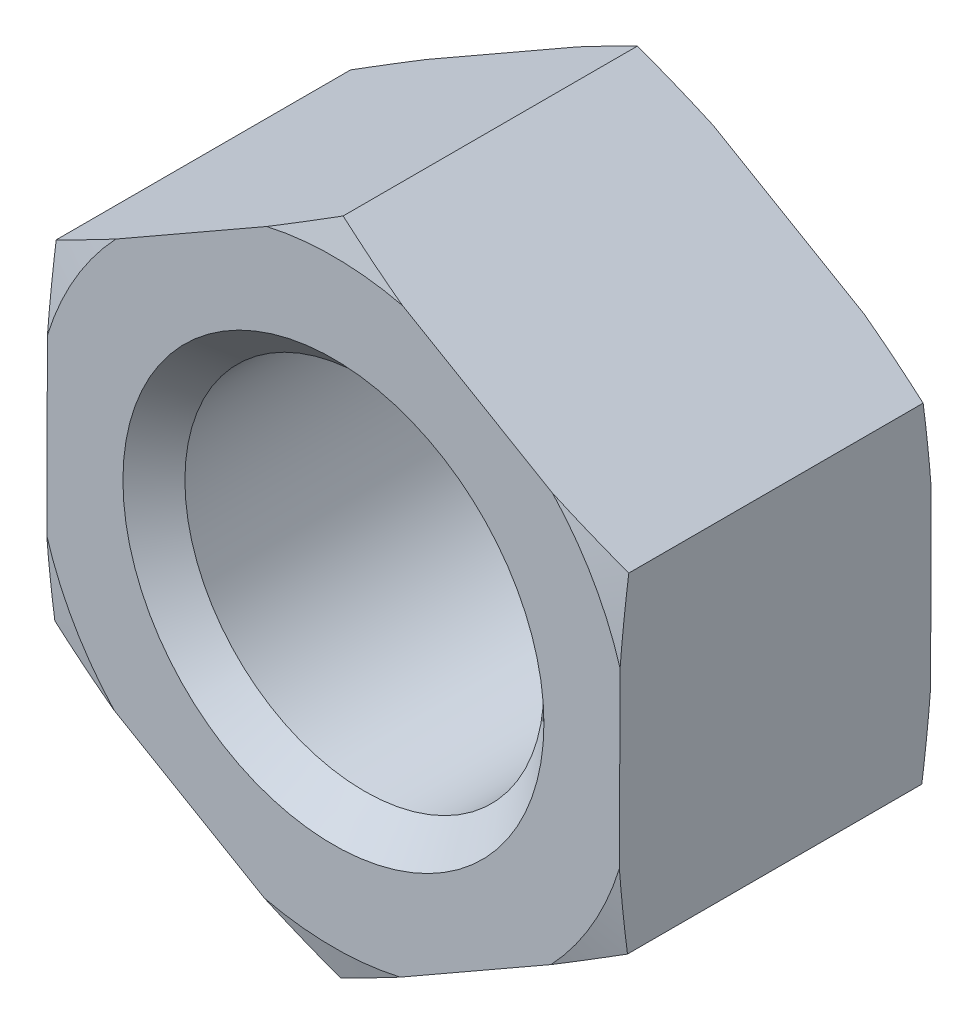
SolidWorks part; units mm, degrees
extrude "Base-Extrude" add sketch "Sketch1" along normal blind 5.2
sketch "Sketch1" plane through (0, 0, 0) normal (0, 0, 1) x (1, 0, 0)
  line L0 (-26.8088, 0) -> (37.1748, 0) construction
  line L1 (0, 25.0215) -> (0, -25.0215) construction
  line L3 (0.0217, 5.525) -> (-4.7739, 2.7813)
  line L4 (-4.7739, 2.7813) -> (-4.7956, -2.7437)
  line L5 (-4.7956, -2.7437) -> (-0.0217, -5.525)
  line L6 (-0.0217, -5.525) -> (4.7739, -2.7813)
  line L7 (4.7739, -2.7813) -> (4.7956, 2.7437)
  line L8 (4.7956, 2.7437) -> (0.0217, 5.525)
  circle A0 centre (0, 0) radius 4.7848 construction
  circle A1 centre (0, 0) radius 3
cosmetic thread "Cosmetic Thread1"
chamfer "Chamfer1" distance 0.5179 angle 45 2 edges at (3, 0, 0) (3, 0, 5.2)
material "  "
ref_plane "Plane1" through (0, 0, 0) normal (0, 0, 1) x (1, 0, 0)
ref_plane "Plane2" through (0, 0, 0) normal (0, 1, 0) x (1, 0, 0)
ref_plane "Plane3" through (0, 0, 0) normal (1, 0, 0) x (0, 0, -1)
sketch "Dimension sketch" plane through (0, 0, 0) normal (0, 0, 1) x (1, 0, 0)
  line L0 (0, 0) -> (30.6749, 0)
  line L1 (30.6749, 0) -> (37.4249, 0)
  line L2 (37.4249, 0) -> (46.3249, 0)
  line L3 (-5.7143, 0) -> (0, 0)
  point P3 (6, 0)
  point P4 (1.5, 0)
  point P5 (11.05, 0)
  point P6 (5.2, 0)
  point P7 (6.4, 0)
  point P8 (10, 0)
sketch "Sketch2" plane through (0, 0, 0) normal (0, 0, -1) x (-1, 0, 0)
  circle A0 centre (0, 0) radius 5
  circle A1 centre (0, 0) radius 3 construction
extrude "Cut-Extrude1" cut sketch "Sketch2" against normal through all draft 75 flip side to cut
sketch "Sketch3" plane through (0, 0, 5.2) normal (0, 0, 1) x (1, 0, 0)
  circle A0 centre (0, 0) radius 5
extrude "Cut-Extrude2" cut sketch "Sketch3" against normal through all draft 75 flip side to cut
equation "\"e@Sketch1\" = \"e@Dimension sketch\""
equation "\"D1@Dimension sketch\" = \"D@Dimension sketch\" / 1.05"
equation "\"D@Sketch1\" = \"D@Dimension sketch\""
equation "\"m@Base-Extrude\" = \"m@Dimension sketch\""
equation "\"D1@Sketch3\" = \"s@Dimension sketch\""
equation "\"s@Sketch2\" = \"s@Dimension sketch\""
equation "\"D2@Cosmetic Thread1\" =\"D@Dimension sketch\""
equation "\"D1@Chamfer1\" =  ( \"da@Dimension sketch\" - \"D1@Dimension sketch\" )  / 2"
